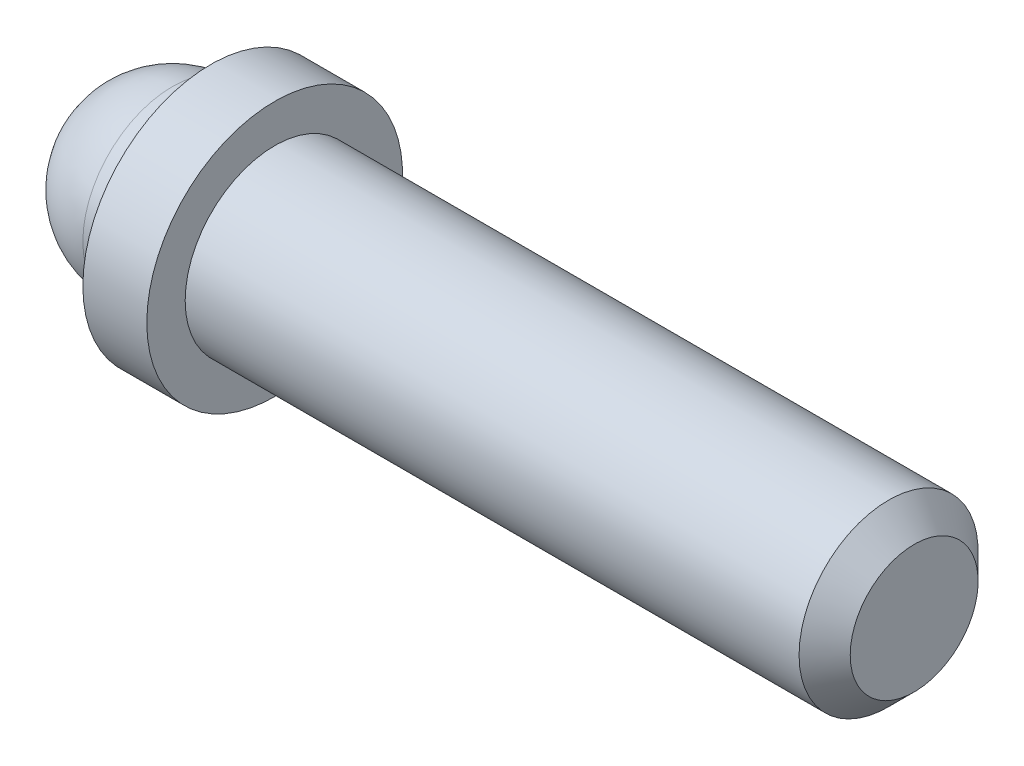
SolidWorks part; units mm, degrees
ref_plane "Front Plane" through (0, 0, 0) normal (0, 0, 1) x (1, 0, 0)
ref_plane "Top Plane" through (0, 0, 0) normal (0, 1, 0) x (1, 0, 0)
ref_plane "Right Plane" through (0, 0, 0) normal (1, 0, 0) x (0, 0, -1)
sketch "Sketch1" plane through (0, 0, 0) normal (0, 0, 1) x (1, 0, 0)
  line L0 (0, 0) -> (0, 5)
  line L1 (-2, 7) -> (-50, 7)
  line L2 (-50, 7) -> (-50, 10)
  line L3 (-50, 10) -> (-55, 10)
  line L4 (-55, 10) -> (-55, 7)
  line L5 (-55, 7) -> (-58, 7)
  line L6 (-89.7586, 0) -> (17.4571, 0) construction
  line L7 (-65, 0) -> (0, 0)
  line L8 (0, 5) -> (-2, 7)
  arc A0 (-65, 0) -> (-58, 7) centre (-58, 0) cw
  point P1 (0, 7)
  dimension "D1" = 5
  dimension "D3" = 65
  dimension "D4" = 7
  dimension "D6" = 10
revolve "Revolve1" add sketch "Sketch1" angle 360 about L6
